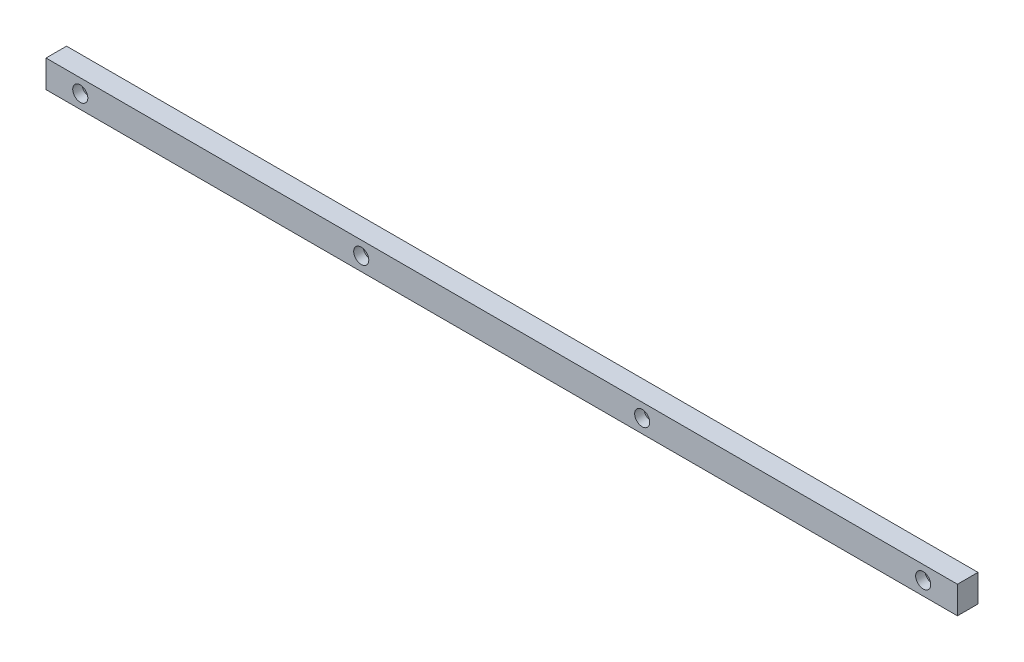
SolidWorks part; units mm, degrees
ref_plane "前视基准面" through (0, 0, 0) normal (0, 0, 1) x (1, 0, 0)
ref_plane "上视基准面" through (0, 0, 0) normal (0, 1, 0) x (1, 0, 0)
ref_plane "右视基准面" through (0, 0, 0) normal (1, 0, 0) x (0, 0, -1)
sketch "草图1" plane through (0, 0, 0) normal (0, 0, 1) x (1, 0, 0)
  line L1 (-332.5, 10) -> (332.5, 10)
  line L2 (-332.5, 10) -> (-332.5, -10)
  line L3 (-332.5, -10) -> (332.5, -10)
  line L4 (332.5, 10) -> (332.5, -10)
  line L5 (-332.5, 10) -> (332.5, -10) construction
  line L6 (-332.5, -10) -> (332.5, 10) construction
  point P0 (0, 0)
  dimension "D1" = 20
  dimension "D2" = 665
extrude "凸台-拉伸1" add sketch "草图1" along normal blind 15
hole_wizard "打孔尺寸(%根据)内六角圆柱头螺钉的类型1" positions "草图2" profile "草图4" counterbore size "M6" standard "GB" end condition through all
sketch "草图2" plane through (0, 0, 15) normal (0, 0, 1) x (1, 0, 0)
  line L0 (-307.5, 0) -> (0, 0) construction
  line L1 (0, 0) -> (307.5, 0) construction
  line L3 (0, 0) -> (0, 67.8719) construction
  point P11 (-307.5, 0)
  point P14 (307.5, 0)
  point P21 (-102.5, 0)
  point P29 (102.5, 0)
  dimension "D1" = 205
  dimension "D2" = 205
sketch "草图4" plane through (102.5, 0, 15) normal (1, 0, 0) x (0, -1, 0)
  line L0 (0, 0) -> (0, 15)
  line L1 (0, 15) -> (3.3, 15)
  line L3 (3.3, 15) -> (3.3, 6.8)
  line L4 (3.3, 6.8) -> (5.5, 6.8)
  line L5 (5.5, 6.8) -> (5.5, 0)
  line L7 (5.5, 0) -> (0, 0)
  line L11 (0, -6.35) -> (0, 107.95) construction
  dimension "通孔孔直径" = 6.6
  dimension "通孔孔深度" = 15
  dimension "柱形沉头孔直径" = 11
  dimension "柱形沉头孔深度" = 6.8
